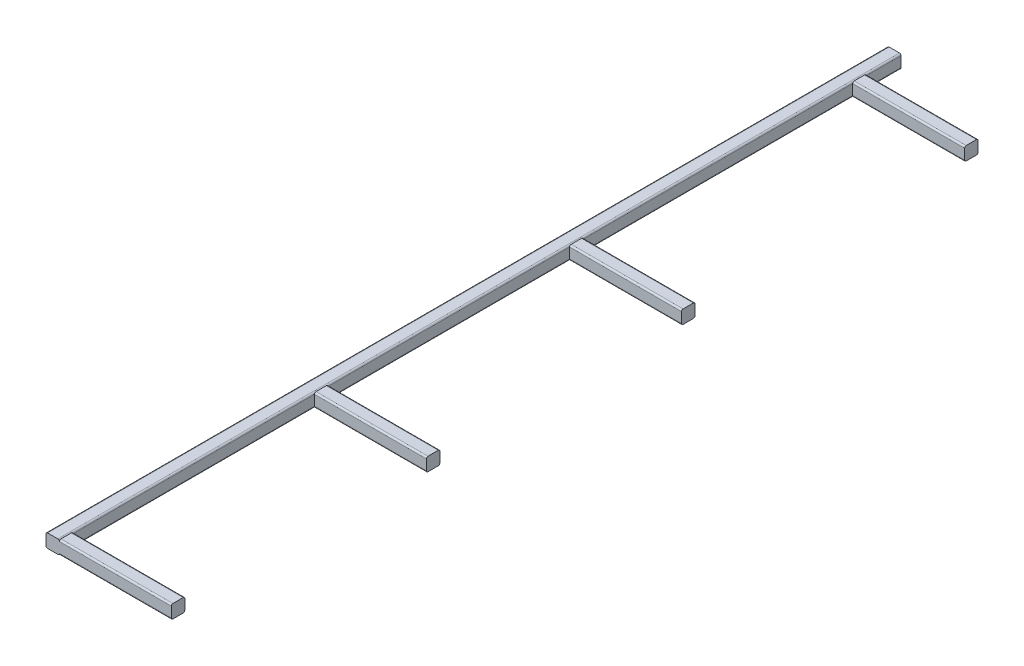
SolidWorks part; units mm, degrees
ref_plane "Front Plane" through (0, 0, 0) normal (0, 0, 1) x (1, 0, 0)
ref_plane "Top Plane" through (0, 0, 0) normal (0, 1, 0) x (1, 0, 0)
ref_plane "Right Plane" through (0, 0, 0) normal (1, 0, 0) x (0, 0, -1)
other "Configuration Table"
sketch "Sketch1" plane through (0, 0, 0) normal (0, 0, 1) x (1, 0, 0)
  line L1 (3.5, 0) -> (26.5, 0)
  line L2 (0, -3.5) -> (0, -26.5)
  line L3 (3.5, -30) -> (26.5, -30)
  line L4 (30, -3.5) -> (30, -26.5)
  arc A0 (26.5, -30) -> (30, -26.5) centre (26.5, -26.5) ccw
  arc A1 (0, -26.5) -> (3.5, -30) centre (3.5, -26.5) ccw
  arc A2 (3.5, 0) -> (0, -3.5) centre (3.5, -3.5) ccw
  arc A3 (26.5, 0) -> (30, -3.5) centre (26.5, -3.5) cw
  point P7 (30, -30)
  point P10 (0, -30)
  point P13 (0, 0)
  point P16 (30, 0)
  dimension "D3" = 3.5
  dimension "D1" = 30
  dimension "D2" = 30
extrude "Boss-Extrude1" add sketch "Sketch1" along normal blind 1880
sketch "Sketch2" plane through (30, 0, 0) normal (1, 0, 0) x (0, 0, -1)
  line L0 (-1880, -30) -> (0, -30) construction
  line L1 (-1876.5, 0) -> (-1853.5, 0)
  line L2 (-1880, -3.5) -> (-1880, -26.5)
  line L3 (-1876.5, -30) -> (-1853.5, -30)
  line L4 (-1850, -3.5) -> (-1850, -26.5)
  line L5 (-1880, 0) -> (0, 0) construction
  line L6 (-104.5615, 0) -> (-81.5615, 0)
  line L7 (-108.0615, -3.5) -> (-108.0615, -26.5)
  line L8 (-104.5615, -30) -> (-81.5615, -30)
  line L9 (-78.0615, -3.5) -> (-78.0615, -26.5)
  line L11 (-1306.7421, 0) -> (-1283.7421, 0)
  line L12 (-1310.2421, -3.5) -> (-1310.2421, -26.5)
  line L13 (-1306.7421, -30) -> (-1283.7421, -30)
  line L14 (-1280.2421, -3.5) -> (-1280.2421, -26.5)
  line L15 (-736.869, 0) -> (-713.869, 0)
  line L16 (-740.369, -3.5) -> (-740.369, -26.5)
  line L17 (-736.869, -30) -> (-713.869, -30)
  line L18 (-710.369, -3.5) -> (-710.369, -26.5)
  arc A0 (-108.0615, -26.5) -> (-104.5615, -30) centre (-104.5615, -26.5) ccw
  arc A1 (-81.5615, -30) -> (-78.0615, -26.5) centre (-81.5615, -26.5) ccw
  arc A2 (-81.5615, 0) -> (-78.0615, -3.5) centre (-81.5615, -3.5) cw
  arc A3 (-104.5615, 0) -> (-108.0615, -3.5) centre (-104.5615, -3.5) ccw
  arc A4 (-736.869, 0) -> (-740.369, -3.5) centre (-736.869, -3.5) ccw
  arc A5 (-740.369, -26.5) -> (-736.869, -30) centre (-736.869, -26.5) ccw
  arc A6 (-713.869, -30) -> (-710.369, -26.5) centre (-713.869, -26.5) ccw
  arc A7 (-713.869, 0) -> (-710.369, -3.5) centre (-713.869, -3.5) cw
  arc A8 (-1306.7421, 0) -> (-1310.2421, -3.5) centre (-1306.7421, -3.5) ccw
  arc A9 (-1310.2421, -26.5) -> (-1306.7421, -30) centre (-1306.7421, -26.5) ccw
  arc A10 (-1283.7421, -30) -> (-1280.2421, -26.5) centre (-1283.7421, -26.5) ccw
  arc A11 (-1283.7421, 0) -> (-1280.2421, -3.5) centre (-1283.7421, -3.5) cw
  arc A12 (-1880, -26.5) -> (-1876.5, -30) centre (-1876.5, -26.5) ccw
  arc A13 (-1853.5, -30) -> (-1850, -26.5) centre (-1853.5, -26.5) ccw
  arc A14 (-1853.5, 0) -> (-1850, -3.5) centre (-1853.5, -3.5) cw
  arc A15 (-1876.5, 0) -> (-1880, -3.5) centre (-1876.5, -3.5) ccw
  point P23 (-108.0615, -30)
  point P26 (-78.0615, -30)
  point P31 (-108.0615, 0)
  point P34 (-740.369, 0)
  point P37 (-740.369, -30)
  point P40 (-710.369, -30)
  point P45 (-1310.2421, 0)
  point P48 (-1310.2421, -30)
  point P51 (-1280.2421, -30)
  point P56 (-1880, -30)
  point P59 (-1850, -30)
  point P64 (-1880, 0)
  dimension "D5" = 3.5
  dimension "D1" = 30
  dimension "D2" = 30
  dimension "D3" = 30
  dimension "D4" = 30
extrude "Boss-Extrude2" add sketch "Sketch2" along normal blind 250
